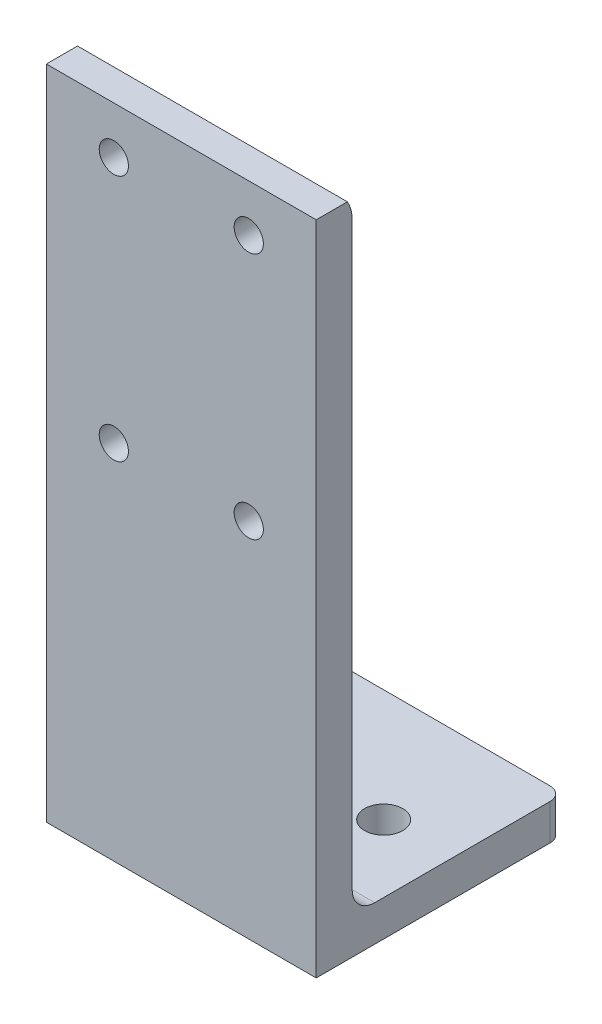
SolidWorks part; units mm, degrees
ref_plane "前视" through (0, 0, 0) normal (0, 0, 1) x (1, 0, 0)
ref_plane "上视" through (0, 0, 0) normal (0, 1, 0) x (1, 0, 0)
ref_plane "右视" through (0, 0, 0) normal (1, 0, 0) x (0, 0, -1)
sketch3d "3D草图1"
  line L0 (0, 0, 0) -> (60, 0, 0)
  dimension "D1" = 60
other "结构构件1"
ref_plane "基准面1" through (0, 0, 0) normal (1, 0, 0) x (0, 0, -1)
sketch "Sketch1" plane through (0, 0, 0) normal (1, 0, 0) x (0, 0, -1)
  line L0 (0, 0) -> (0, 150)
  line L1 (0, 75) -> (8, 75) construction
  line L2 (8, 142) -> (8, 13)
  line L3 (13, 8) -> (62, 8)
  line L4 (35, 8) -> (35, 0) construction
  line L5 (70, 0) -> (0, 0)
  arc A0 (70, 0) -> (62, 8) centre (62, 0) ccw
  arc A1 (0, 150) -> (8, 142) centre (0, 142) cw
  arc A2 (13, 8) -> (8, 13) centre (13, 13) cw
  point P10 (35, 0)
  point P14 (0, 75)
  point P15 (8, 75)
  point P16 (35, 8)
  point P17 (0, 0)
  dimension "D2" = 8
  dimension "D3" = 70
  dimension "Radius_1" = 5
  dimension "D1" = 8
  dimension "D4" = 150
sketch "草图3" plane through (0, 0, 0) normal (0, -1, 0) x (1, 0, 0)
  line L0 (60, 0) -> (60, -70) construction
  line L1 (0, -70) -> (60, -70)
  line L2 (0, -70) -> (0, -55)
  line L3 (0, -55) -> (60, -55)
  line L4 (60, -70) -> (60, -55)
  line L5 (60, -70) -> (0, -70) construction
  dimension "D1" = 15
extrude "切除-拉伸1" cut sketch "草图3" against normal through all
sketch "草图4" plane through (0, 0, 0) normal (0, 0, 1) x (1, 0, 0)
  line L0 (0, 150) -> (0, 0) construction
  line L1 (60, 150) -> (0, 150)
  line L2 (60, 150) -> (60, 146)
  line L3 (60, 146) -> (0, 146)
  line L4 (0, 150) -> (0, 146)
  dimension "D1" = 4
extrude "切除-拉伸2" cut sketch "草图4" against normal through all
hole_wizard "Ø6.5 (6.5) 直径孔1" positions "草图6" profile "草图5" hole size "Ø6.5" standard "GB" end condition through all
sketch "草图6" plane through (0, 0, -8) normal (0, 0, -1) x (-1, 0, 0)
  line L0 (-30, 0) -> (-30, 127.317) construction
  line L1 (-60, 0) -> (0, 0) construction
  line L3 (0, 146) -> (-60, 146) construction
  point P0 (-45, 135.5)
  point P3 (-15, 135.5)
  point P5 (-45, 80.5)
  point P8 (-15, 80.5)
  dimension "D1" = 30
  dimension "D2" = 55
  dimension "D3" = 10.5
sketch "草图5" plane through (45, 135.5, -8) normal (1, 0, 0) x (0, 1, 0)
  line L0 (0, 0) -> (0, 8)
  line L1 (0, 8) -> (3.25, 8)
  line L2 (3.25, 8) -> (3.25, 0)
  line L5 (3.25, 0) -> (0, 0)
  line L11 (0, -6.35) -> (0, 107.95) construction
  dimension "通孔孔直径" = 6.5
  dimension "通孔孔深度" = 8
fillet "圆角1" radius 3 2 edges at (0, 4, -55) (60, 4, -55)
hole_wizard "Ø8.5 (8.5) 直径孔1" positions "草图7" profile "草图8" hole size "Ø8.5" standard "GB" end condition through all
sketch "草图7" plane through (0, 8, 0) normal (0, 1, 0) x (1, 0, 0)
  line L0 (30, 0) -> (30, 67.6894) construction
  line L1 (0, 0) -> (60, 0) construction
  line L3 (57, 55) -> (3, 55) construction
  point P0 (15, 30)
  point P2 (45, 30)
  dimension "D1" = 25
  dimension "D2" = 30
sketch "草图8" plane through (15, 8, -30) normal (1, 0, 0) x (0, 0, 1)
  line L0 (0, 0) -> (0, 8)
  line L1 (0, 8) -> (4.25, 8)
  line L2 (4.25, 8) -> (4.25, 0)
  line L5 (4.25, 0) -> (0, 0)
  line L11 (0, -6.35) -> (0, 107.95) construction
  dimension "通孔孔直径" = 8.5
  dimension "通孔孔深度" = 8
